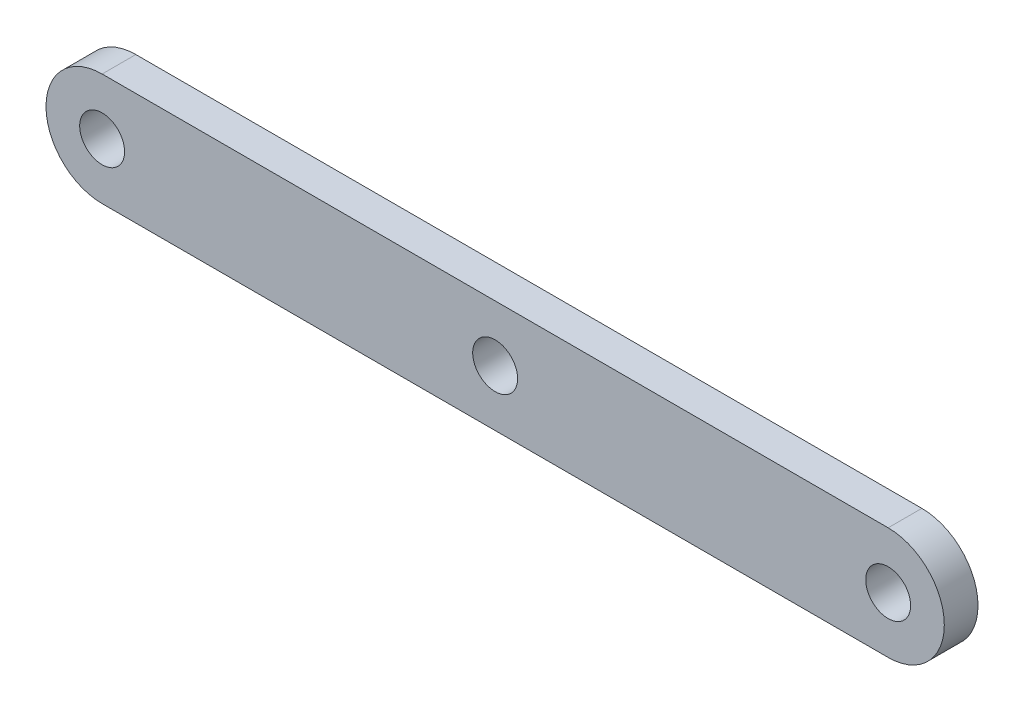
from build123d import *

# Parameters (mm, degrees)
BOSS_EXTRUDE1_DEPTH = 6
SKETCH2_R           = 4
CUT_EXTRUDE1_DEPTH  = 95
SKETCH3_R           = 4
CUT_EXTRUDE2_DEPTH  = 10


with BuildPart() as part:
    # Sketch1 → Boss-Extrude1 (new body)
    with BuildSketch(Plane.XY):
        with BuildLine():
            Line((0, 10), (140, 10))
            ThreePointArc((140, 10), (150, 0), (140, -10))
            Line((140, -10), (0, -10))
            ThreePointArc((0, -10), (-10, 0), (0, 10))
        make_face()
    extrude(amount=BOSS_EXTRUDE1_DEPTH)

    # Sketch2 → Cut-Extrude1 (cut)
    with BuildSketch(Plane.XY.offset(6)):
        Circle(SKETCH2_R)
        with Locations((140, 0)):
            Circle(SKETCH2_R)
    extrude(amount=-CUT_EXTRUDE1_DEPTH, mode=Mode.SUBTRACT)

    # Sketch3 → Cut-Extrude2 (cut)
    with BuildSketch(Plane.XY.offset(6)):
        with Locations((70, 0)):
            Circle(SKETCH3_R)
    extrude(amount=-CUT_EXTRUDE2_DEPTH, mode=Mode.SUBTRACT)


solid = part.part
